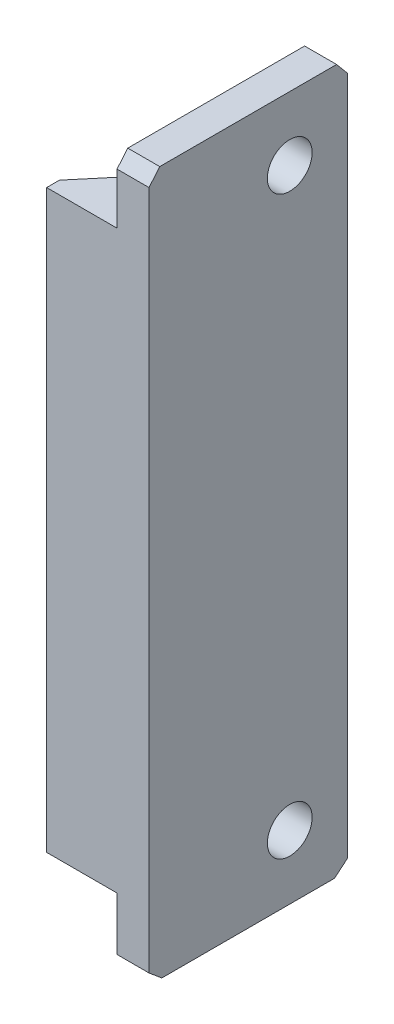
from build123d import *
from OCP.BRepFilletAPI import BRepFilletAPI_MakeChamfer

# Parameters (mm, degrees)
SKETCH1_W           = 8
SKETCH1_H           = 15.5
BOSS_EXTRUDE1_DEPTH = 55
SKETCH2_W           = 5.5
SKETCH2_H           = 11.5
CUT_EXTRUDE1_DEPTH  = 58.699653379
CHAMFER1_SIZE       = 3
CHAMFER1_SIZE2      = 2.517298894
SKETCH3_R           = 1.75
CUT_EXTRUDE2_DEPTH  = 48
SKETCH4_W           = 5.5
SKETCH4_H           = 5
CUT_EXTRUDE3_DEPTH  = 57.756056945
CHAMFER2_SIZE       = 1
CHAMFER2_SIZE2      = 0.839099631


with BuildPart() as part:
    # Sketch1 → Boss-Extrude1 (new body)
    with BuildSketch(Plane(origin=(0, 0, 0), x_dir=(1, 0, 0), z_dir=(0, 1, 0))):
        with Locations((4, 7.75)):
            Rectangle(SKETCH1_W, SKETCH1_H)
    extrude(amount=BOSS_EXTRUDE1_DEPTH)

    # Sketch2 → Cut-Extrude1 (cut, through all)
    with BuildSketch(Plane(origin=(0, 55, 0), x_dir=(1, 0, 0), z_dir=(0, 1, 0))):
        with Locations((2.75, 9.75)):
            Rectangle(SKETCH2_W, SKETCH2_H)
    extrude(amount=-CUT_EXTRUDE1_DEPTH, mode=Mode.SUBTRACT)

    # Chamfer1
    chamfer1_edges = [part.edges().sort_by_distance(p)[0] for p in [
        (0, 27.5, -4),
    ]]
    chamfer1_side = [part.faces().sort_by_distance(p)[0] for p in [
        (0, 27.5, -2),
    ]]
    chamfer(chamfer1_edges, length=CHAMFER1_SIZE, length2=CHAMFER1_SIZE2, reference=chamfer1_side[0])

    # Sketch3 → Cut-Extrude2 (cut)
    with BuildSketch(Plane(origin=(8, 0, 0), x_dir=(0, 0, -1), z_dir=(1, 0, 0))):
        with Locations((11, 50)):
            Circle(SKETCH3_R)
        with Locations((11, 5)):
            Circle(SKETCH3_R)
    extrude(amount=-CUT_EXTRUDE2_DEPTH, mode=Mode.SUBTRACT)

    # Sketch4 → Cut-Extrude3 (cut, through all)
    with BuildSketch(Plane(origin=(0, 0, -4), x_dir=(-1, 0, 0), z_dir=(0, 0, -1))):
        with Locations((-2.75, 52.5)):
            Rectangle(SKETCH4_W, SKETCH4_H)
        with Locations((-2.75, 2.5)):
            Rectangle(SKETCH4_W, SKETCH4_H)
    extrude(amount=-CUT_EXTRUDE3_DEPTH, mode=Mode.SUBTRACT)

    # Chamfer2: one chamfer whose edges measure the first distance from different faces: ONE call of the kernel's chamfer builder (chamfer() names one face for all edges)
    chamfer2_edges_1 = [part.edges().sort_by_distance(p)[0] for p in [
        (6.75, 55, -15.5),
    ]]
    chamfer2_side_1 = [part.faces().sort_by_distance(p)[0] for p in [
        (6.75, 27.5, -15.5),
    ]]
    chamfer2_edges_2 = [part.edges().sort_by_distance(p)[0] for p in [
        (6.75, 0, -15.5),
        (6.75, 0, 0),
    ]]
    chamfer2_side_2 = [part.faces().sort_by_distance(p)[0] for p in [
        (6.75, 0, -7.75),
    ]]
    chamfer2_edges_3 = [part.edges().sort_by_distance(p)[0] for p in [
        (6.75, 55, 0),
    ]]
    chamfer2_side_3 = [part.faces().sort_by_distance(p)[0] for p in [
        (4.178571429, 27.5, 0),
    ]]
    chamfer2 = BRepFilletAPI_MakeChamfer(part.part.solid().wrapped)
    for e in chamfer2_edges_1:
        chamfer2.Add(CHAMFER2_SIZE, CHAMFER2_SIZE2, e.wrapped, chamfer2_side_1[0].wrapped)  # the first distance lies on this face
    for e in chamfer2_edges_2:
        chamfer2.Add(CHAMFER2_SIZE, CHAMFER2_SIZE2, e.wrapped, chamfer2_side_2[0].wrapped)  # the first distance lies on this face
    for e in chamfer2_edges_3:
        chamfer2.Add(CHAMFER2_SIZE, CHAMFER2_SIZE2, e.wrapped, chamfer2_side_3[0].wrapped)  # the first distance lies on this face
    add(Compound.cast(chamfer2.Shape()), mode=Mode.REPLACE)


solid = part.part
